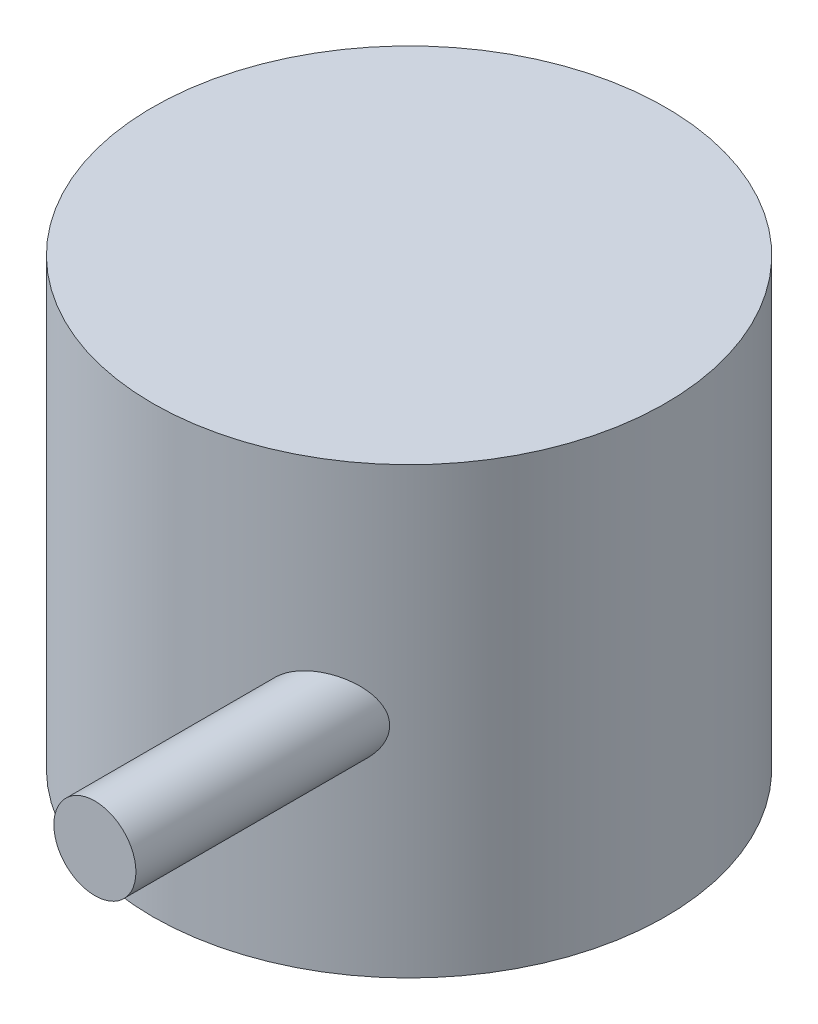
SolidWorks part; units mm, degrees
ref_plane "Front Plane" through (0, 0, 0) normal (0, 0, 1) x (1, 0, 0)
ref_plane "Top Plane" through (0, 0, 0) normal (0, 1, 0) x (1, 0, 0)
ref_plane "Right Plane" through (0, 0, 0) normal (1, 0, 0) x (0, 0, -1)
sketch "Sketch1" plane through (0, 0, 0) normal (0, 1, 0) x (1, 0, 0)
  circle A0 centre (0, 0) radius 37.5
  dimension "D1" = 75
extrude "Boss-Extrude1" add sketch "Sketch1" along normal blind 65
sketch "Sketch2" plane through (0, 0, 0) normal (0, 0, 1) x (1, 0, 0)
  line L0 (-37.5, 65) -> (-37.5, 0) construction
  circle A0 centre (19.06, 31.9334) radius 6
  dimension "D1" = 12
  dimension "D2" = 56.56
extrude "Boss-Extrude2" add sketch "Sketch2" along normal blind 65
